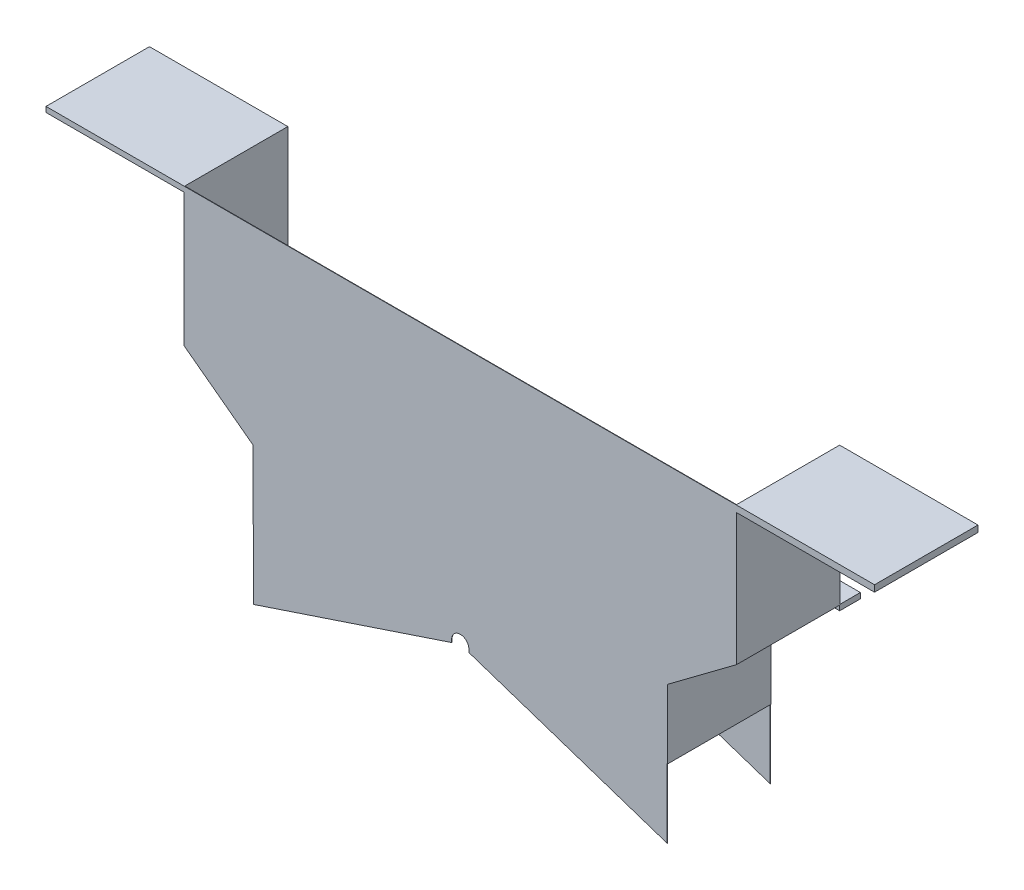
from build123d import *

# Parameters (mm, degrees)
EXTRUDE_1_DEPTH     = 0.6
EXTRUDE_2_DEPTH     = 150
EXTRUDE_START       = -0.6
EXTRUDE_3_DEPTH     = 0.6
EXTRUDE_4_DEPTH     = 0.6
CUT_EXTRUDE_1_DEPTH = 569.863461773
EXTRUDE_5_DEPTH     = 100
SKETCH_9_W          = 150
SKETCH_9_H          = 7.683379221
EXTRUDE_6_DEPTH     = 200
SKETCH_11_W         = 150
SKETCH_11_H         = 9.400930001
EXTRUDE_7_DEPTH     = 200
EXTRUDE_10_DEPTH    = 2
SKETCH_16_W         = 799.99994366
SKETCH_16_H         = 30
EXTRUDE_12_DEPTH    = 8


with BuildPart() as part:
    # 草图1 → 凸台-拉伸1 (new body)
    with BuildSketch(Plane.XY):
        with BuildLine():
            Line((300, 0), (300, 230))
            Line((300, 230), (-300, 230))
            Line((-300, 230), (-300, 0))
            Line((-300, 0), (-9.486832981, 96.83772234))
            ThreePointArc((-9.486832981, 96.83772234), (0, 110), (9.486832981, 96.83772234))
            Line((9.486832981, 96.83772234), (300, 0))
        make_face()
    extrude(amount=EXTRUDE_1_DEPTH)

    # 草图4 → 凸台-拉伸2 (add)
    with BuildSketch(Plane(origin=(0, 0, 0), x_dir=(-1, 0, 0), z_dir=(0, 0, -1))):
        Polygon((-400, 375), (-400, 275), (-300, 200.300723127), (-300, 200), (-300, 100), (-300.6, 100), (-300.6, 200), (-400.600347155, 274.699536196), (-400.600347155, 375), align=None)
        Polygon((300, 100), (300.6, 100), (300.6, 200), (400.600347155, 274.699536196), (400.600347155, 375), (400, 375), (400, 275), (300, 200.300723127), (300, 200), align=None)
    extrude(amount=-EXTRUDE_2_DEPTH)

    # 草图5 → 凸台-拉伸3 (add)
    with BuildSketch(Plane.XY.offset(150).offset(EXTRUDE_START)):
        with BuildLine():
            Line((-300, 0), (-300, 100))
            Line((-300, 100), (-300.6, 100))
            Line((-300.6, 100), (-300.6, 200))
            Line((-300.6, 200), (-400.600347155, 274.699536196))
            Line((-400.600347155, 274.699536196), (-400.600347155, 375))
            Line((-400.600347155, 375), (400.600347155, 375))
            Line((400.600347155, 375), (400.600347155, 274.699536196))
            Line((400.600347155, 274.699536196), (300.6, 200))
            Line((300.6, 200), (300.6, 115))
            Line((300.6, 115), (300, 115))
            Line((300, 115), (300, 0))
            Line((300, 0), (9.486832981, 96.83772234))
            ThreePointArc((9.486832981, 96.83772234), (0, 110), (-9.486832981, 96.83772234))
            Line((-9.486832981, 96.83772234), (-300, 0))
        make_face()
    extrude(amount=EXTRUDE_3_DEPTH)

    # 草图6 → 凸台-拉伸4 (add)
    with BuildSketch(Plane(origin=(0, 0, 0), x_dir=(-1, 0, 0), z_dir=(0, 0, -1))):
        with BuildLine():
            Line((-300, 230), (-340.599999933, 230))
            Line((-340.599999933, 230), (-300.6, 200))
            ThreePointArc((-300.6, 200), (-300.207294902, 199.964589803), (-300, 200.3))
            Line((-300, 200.3), (-300, 230))
        make_face()
        Polygon((300, 230), (343.651844708, 232.159416678), (300.6, 200), (300, 200.300723127), align=None)
    extrude(amount=-EXTRUDE_4_DEPTH)

    # 草图7 → 切除-拉伸1 (cut, through all)
    with BuildSketch(Plane.XY.offset(150)):
        with BuildLine():
            Line((-12.5, 100), (-12.5, 86.103683602))
            Line((-12.5, 86.103683602), (12.5, 86.103683602))
            Line((12.5, 86.103683602), (12.5, 100))
            ThreePointArc((12.5, 100), (0, 112.5), (-12.5, 100))
        make_face()
    extrude(amount=-CUT_EXTRUDE_1_DEPTH, mode=Mode.SUBTRACT)

    # 草图8 → 凸台-拉伸5 (add)
    with BuildSketch(Plane(origin=(0, 375, 0), x_dir=(1, 0, 0), z_dir=(0, 1, 0))):
        Polygon((-400.600347155, 0), (-400, 0), (-400, -149.4), (400, -149.4), (400, 0), (400.600347155, 0), (400.600347155, -149.4), (400.600347155, -150), (-400, -150), (-400.600347155, -150), align=None)
    extrude(amount=EXTRUDE_5_DEPTH)

    # 草图9 → 凸台-拉伸6 (add)
    with BuildSketch(Plane.ZY.offset(400.600347155)):
        with Locations((75, 471.15831039)):
            Rectangle(SKETCH_9_W, SKETCH_9_H)
    extrude(amount=EXTRUDE_6_DEPTH)

    # 草图11 → 凸台-拉伸7 (add)
    with BuildSketch(Plane(origin=(400.600347155, 0, 0), x_dir=(0, 0, -1), z_dir=(1, 0, 0))):
        with Locations((-75, 470.299535)):
            Rectangle(SKETCH_11_W, SKETCH_11_H)
    extrude(amount=EXTRUDE_7_DEPTH)

    # 草图12 → 凸台-拉伸10 (add)
    with BuildSketch(Plane(origin=(0, 0, 0), x_dir=(-1, 0, 0), z_dir=(0, 0, -1))):
        Polygon((-339.758452982, 230), (-400, 275), (400.600347155, 274.699536196), (342.578162478, 232.106302604), align=None)
    extrude(amount=-EXTRUDE_10_DEPTH)

    # 草图16 → 凸台-拉伸12 (add)
    with BuildSketch(Plane(origin=(-0.103150629, 274.84984204, 0), x_dir=(0.9999999295756685, 0.00037529809229504854, 0), z_dir=(-0.0003752980922950485, 0.9999999295756684, 0))):
        with Locations((0.178266594, 15)):
            Rectangle(SKETCH_16_W, SKETCH_16_H)
    extrude(amount=-EXTRUDE_12_DEPTH)


solid = part.part
